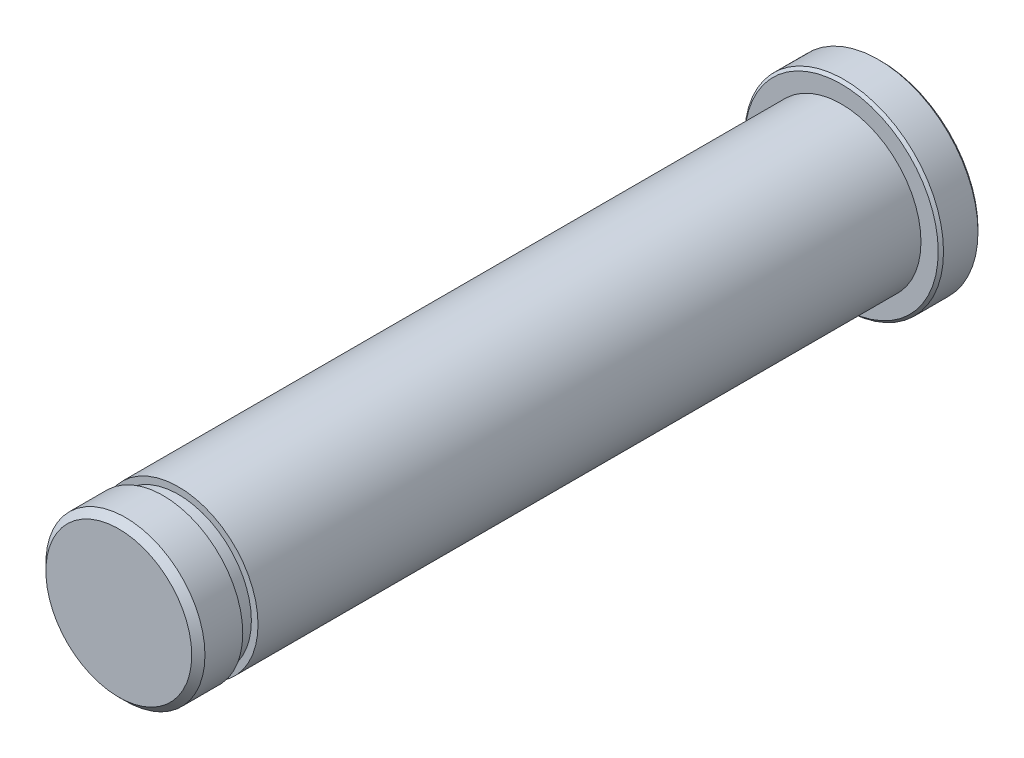
from build123d import *

# Parameters (mm, degrees)
SKETCH1_R           = 7.5
BOSS_EXTRUDE1_DEPTH = 3
SKETCH2_R           = 6
BOSS_EXTRUDE2_DEPTH = 54.5
CHAMFER1_SIZE       = 0.2
SKETCH3_W           = 0.5
SKETCH3_H           = 1.15
CHAMFER2_SIZE       = 0.5


with BuildPart() as part:
    # Sketch1 → Boss-Extrude1 (new body)
    with BuildSketch(Plane.XY):
        Circle(SKETCH1_R)
    extrude(amount=BOSS_EXTRUDE1_DEPTH)

    # Sketch2 → Boss-Extrude2 (add)
    with BuildSketch(Plane.XY.offset(3)):
        Circle(SKETCH2_R)
    extrude(amount=BOSS_EXTRUDE2_DEPTH)

    # Chamfer1
    chamfer1_edges = [part.edges().sort_by_distance(p)[0] for p in [
        (-7.5, 0, 0),
        (-7.5, 0, 3),
    ]]
    chamfer(chamfer1_edges, length=CHAMFER1_SIZE)

    # Sketch3 → Cut-Revolve1 (revolve, cut)
    with BuildSketch(Plane(origin=(0, 0, 0), x_dir=(1, 0, 0), z_dir=(0, 1, 0)), mode=Mode.PRIVATE) as cut_revolve1_sk:
        with Locations((-5.75, -53.575)):
            Rectangle(SKETCH3_W, SKETCH3_H)
    revolve(cut_revolve1_sk.sketch.rotate(Axis((0, 0, 57.5), (0, 0, -1)), 180), axis=Axis((0, 0, 57.5), (0, 0, -1)), mode=Mode.SUBTRACT)

    # Chamfer2
    chamfer2_edges = [part.edges().sort_by_distance(p)[0] for p in [
        (-6, 0, 57.5),
    ]]
    chamfer(chamfer2_edges, length=CHAMFER2_SIZE)


solid = part.part
